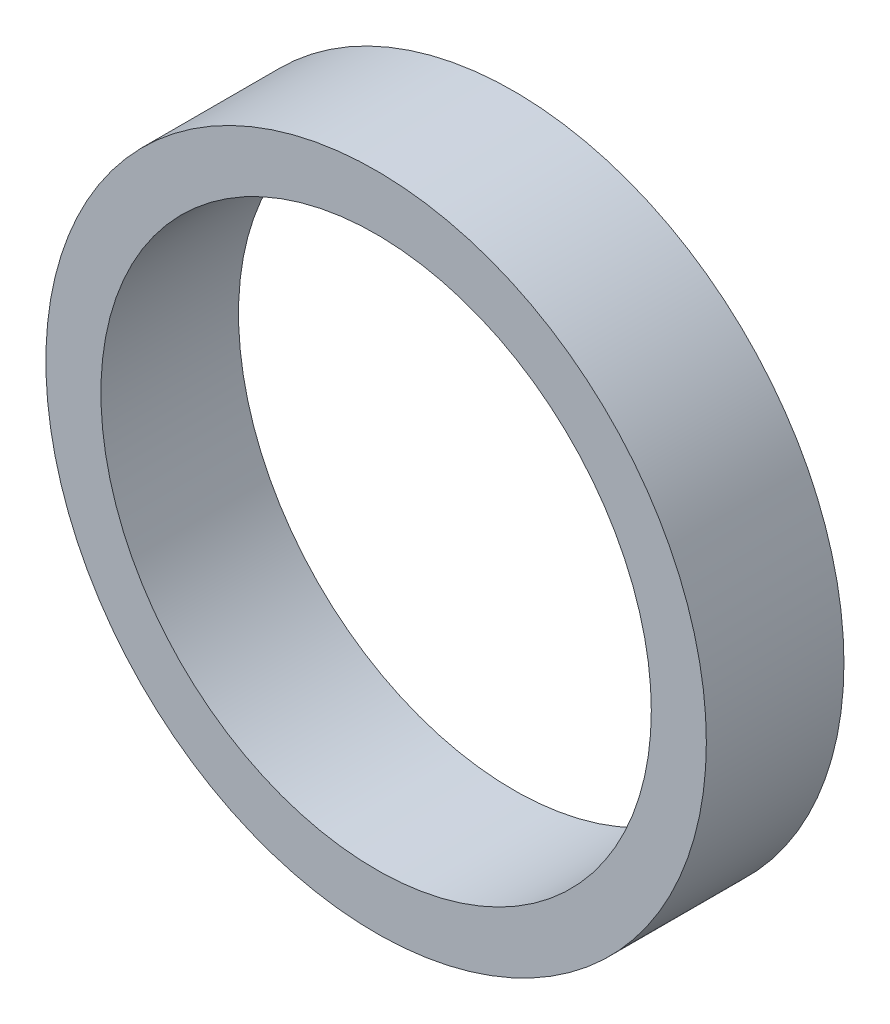
from build123d import *

# Parameters (mm, degrees)
SKETCH_2_R      = 24
SKETCH_2_R_2    = 20
EXTRUDE_1_DEPTH = 10


with BuildPart() as part:
    # 草图2 → 凸台-拉伸1 (new body)
    with BuildSketch(Plane.XY):
        Circle(SKETCH_2_R)
        Circle(SKETCH_2_R_2, mode=Mode.SUBTRACT)
    extrude(amount=EXTRUDE_1_DEPTH)


solid = part.part
